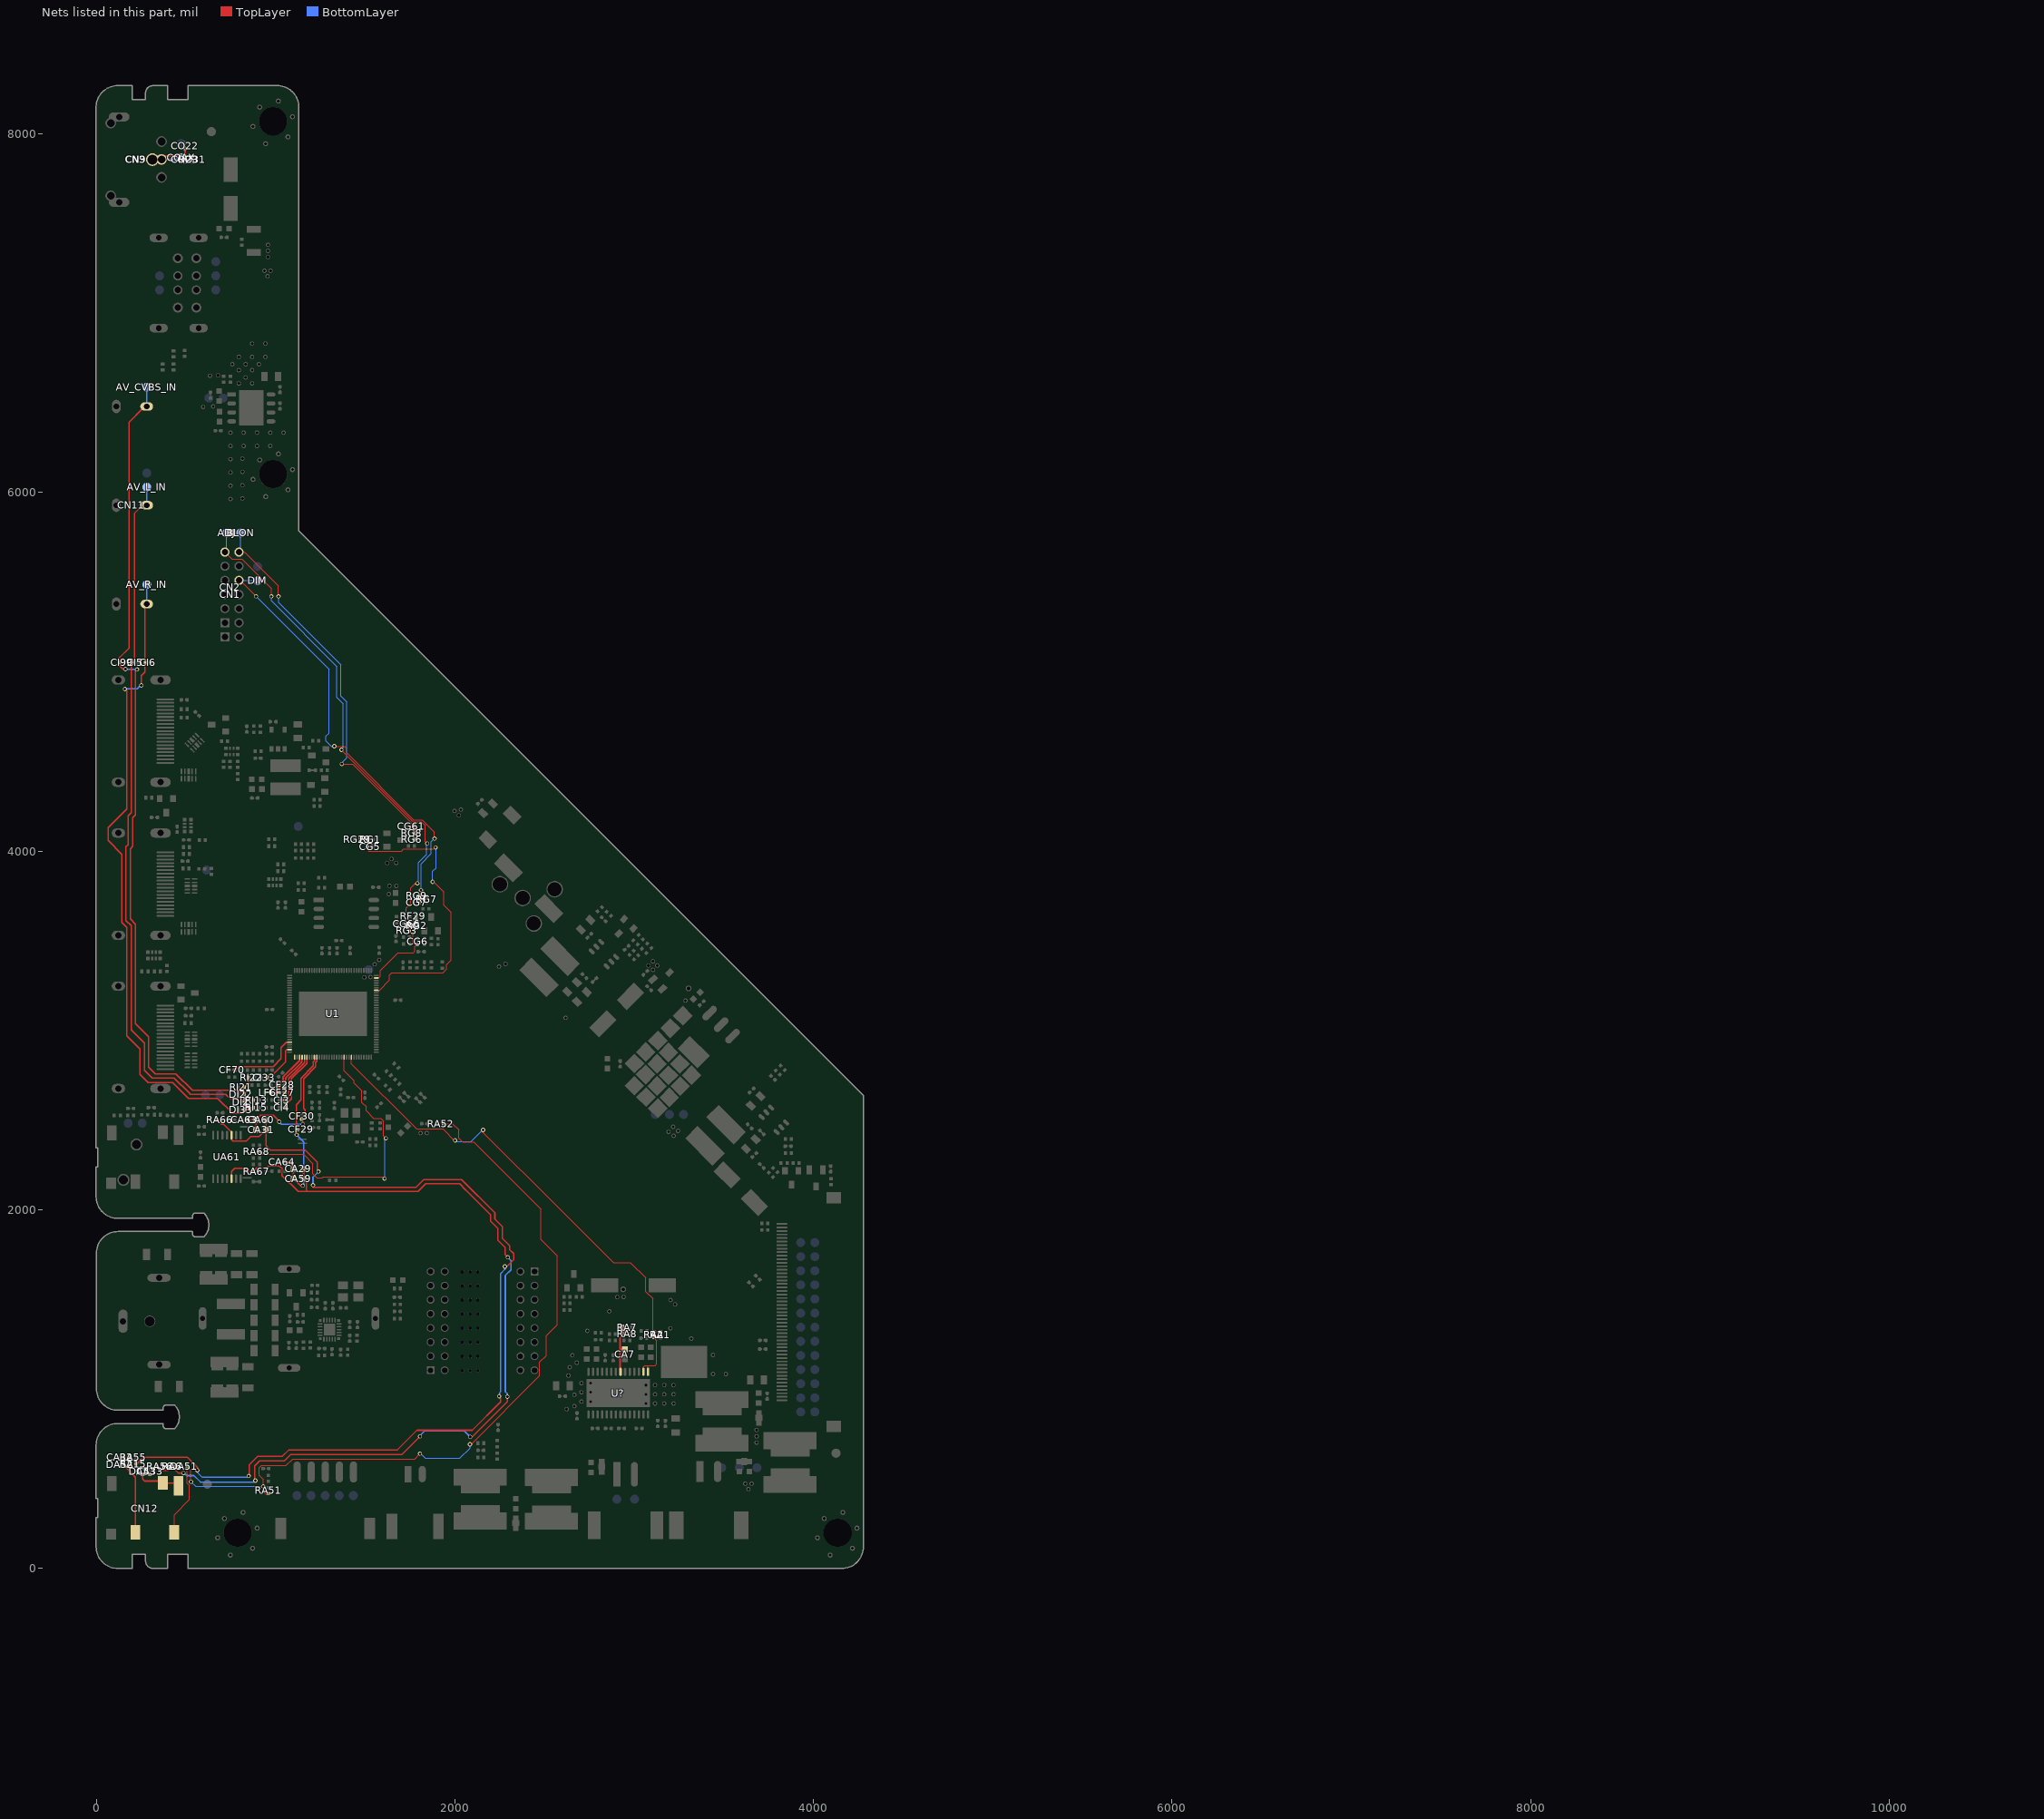
[diagram p0: the nets of this part, all layers, seen from the top]
# Altium PCB MISC105950.PcbDoc (part 6 of 15)
Units mil, origin at the board's own origin, x right, y up, seen from the top; angles counter-clockwise.
Board outline 4280.62 x 8272.76 mil, 2 copper layers (TopLayer, BottomLayer), stack 61.855 mil thick; 541 components, 268 nets, 2324 pads, 1157 vias.

## Via types
v1: diameter 23.62, hole 15.75, TopLayer to BottomLayer, tented both sides, 1087 vias
v2: diameter 23.62, hole 15.75, TopLayer to BottomLayer, 51 vias
v3: diameter 27.56, hole 19.68, TopLayer to BottomLayer, 15 vias
v4: diameter 31.5, hole 19.68, TopLayer to BottomLayer, tented both sides, 4 vias

## Nets (pads, with @x,y where several pads share a name; then routed paths per layer and width w, separated by ;. In a path a pad name is that pad's centre, name@x,y a point inside that pad or via, vN(x,y) a via of type N, cw(c..) or ccw(c..) an arc to the next point about the centre after c; other vN are vias at no path point) (continued)
ADIM: CG7.2@1795.85,3714 CG7.2@1802.74,3714 CN1.10 CN2.8 DIM.1 RG7.1 RG9.2 | length 2514.3
  TopLayer w5: CN2.8@794.34,5510.06 799.94,5510.06 v1(889.5,5420.5) ; v1(1326.5,4584.5) 1382,4584.5 1393.5,4573 1393.5,4549.61 1769.11,4174 1815.14,4174 1885,4104.14 v1@1885,4072 ; CG7.2@1802.74,3714 1803.23,3714.5 RG9.2@1803.23,3752 ; v1(1810,3782) 1810,3752 RG9.2@1803.23,3752 ; RG7.1@1841,3747.23 1836.23,3752 RG9.2@1803.23,3752
  BottomLayer w5: CN2.8@794.34,5510.06 897.01,5510.06 DIM.1@898.43,5508.64 ; v1(889.5,5420.5) 1296.5,5013.5 1296.5,4657.37 1279.69,4640.56 1279.69,4614.81 1310,4584.5 v1(1326.5,4584.5) ; v1(1810,3782) 1810,3928.5 1866.96,3985.46 1866.96,4050.96 v1(1885.5,4069.5)
ADIM_OUT_IC: CG5.2@1508.76,4024 CG5.2@1515.65,4024 RG1.2 RG29.1 U1.90 | length 1687
  TopLayer w5: RG29.1@1472.23,4064.5 RG1.2@1510.77,4064.5 CG5.2@1510.77,4026 ; CG5.2@1508.76,4024 1508.76,4008.24 1517,4000 1701.36,4000 1711.86,4010.5 1882,4010.5 v1(1891.5,4020) ; U1.90@1560.66,3222.78 1577.7,3222.78 1633.94,3279.02 1633.94,3293.19 1633.94,3309.19 1645.25,3320.5 1694.91,3320.5 1695,3320.4 1724,3320.4 1724.09,3320.5 1931.54,3320.5 1952.5,3341.46 1952.5,3365.22 1978.31,3391.03 1978.31,3656.47 1936.5,3698.28 1936.5,3771.14 1879.14,3828.5 v1(1874.5,3828.5) v1@1874.56,3828.44
  BottomLayer w5: v1(1874.5,3828.5) 1874.5,3886.5 1893.31,3905.31 v1@1893.31,4018.19
ADJ/PWM: ADJ.1 CG66.2@1738.85,3595 CG66.2@1745.74,3595 CN1.13 CN2.11 RG3.1 | length 2856.5
  TopLayer w5: CN2.11@715.6,5667.54 754.65,5628.5 812,5628.5 975,5465.5 v1(975,5420.5) ; v1@1366,4562.96 1764.96,4164 1811,4164 1832.69,4142.31 1832.69,4051.31 v1@1848,4036 ; RG3.1@1745.73,3555.5 CG66.2@1745.74,3595 1745.74,3611.22 1728.5,3628.46 1728.5,3682 1752.91,3706.41 1752.91,3787.5 1753.19,3787.77 1753.19,3793.5 ; v1@1789,3819.5 1779.19,3819.5 1753.19,3793.5 ; v1(1789.5,3820) 1789.5,3829.81 1753.19,3793.5
  BottomLayer w5: CN2.11@724.76,5676.7 ADJ.1@724.76,5772.46 ; v1(975,5420.5) 975,5396.52 1341.28,5030.24 1341.28,4856.91 1375.5,4822.69 1375.5,4576.5 v1@1366,4567 ; v1@1796,3826.5 1796,3935 1842.5,3981.5 v1@1842.5,4039.84
  other v1: 1844.5,4042 1366,4565
AMP_L_OUT_IC: CA29.1 CA59.1 CA64.1 CF29.1 U1.41 | length 1132.5
  TopLayer w7: CA64.1@1051.73,2262.41 CA64.1@1051.73,2266 1091.5,2266 1098.17,2259.33 CA29.1@1098.17,2226.34 CA59.1@1098.17,2172.75 1137.92,2133 v1(1150.5,2133) ; v1(1116,2416.5) 1113.69,2418.81 1113.69,2584.75 1140,2611.06 1140,2731 1209.82,2800.82 1209.82,2824.18 1215.15,2829.52 U1.41@1215.15,2849.72
  BottomLayer w7: v1(1116,2416.5) 1154.5,2378 1154.5,2301 ; v1(1150.5,2133) 1154.5,2137 1154.5,2186.5 ; 1154.5,2174.5 1154.5,2186.5 ; 1154.5,2192.5 1154.5,2301 ; 1154.5,2327.5 1154.5,2301 ; 1154.5,2186.5 1154.5,2301
AMP_MUTE_OUT: RA2.1 U?.1 U?.2 | length 295
  TopLayer w5: U?.2@3050.95,1094.5 3050.95,1122.45 3057.94,1129.44 3115.94,1129.44 3125.5,1139 3125.5,1268.27 RA2.1@3109,1284.77 ; U?.1@3076.54,1094.5 3076.54,1127.5
AMP_MUTE_OUT_IC: RA1.1 RA2.2 U1.56 | length 2607.4
  TopLayer w5: U1.56@1421.85,2849.72 1421.85,2812.98 1785.83,2449 1931.5,2449 v1@1997.5,2383 ; v1(2156,2444) 2156,2430.59 2584.34,2002.25 2585.91,2002.25 2883.67,1704.5 2978.7,1704.5 3063,1620.2 3063,1542.5 3102.95,1502.55 3102.95,1401.5 ; 3102.95,1373.86 3102.95,1401.5 ; RA1.1@3145,1318.23 RA2.2@3109,1318.23 3102.95,1324.28 3102.95,1401.5
  BottomLayer w5: v1@2007,2378.5 2090.5,2378.5 v1(2156,2444)
  other v1: 2000,2385.5
AMP_R_OUT_IC: CA31.1 CA60.1 CA63.1 CF30.1 U1.42 | length 829.4
  TopLayer w7: CA63.1@841.5,2501 888.56,2501 CA60.1@889.56,2500 ; CA60.1@889.31,2499.75 CA60.1@889.56,2500 ; CA31.1@889.81,2445 889.81,2499.75 CA60.1@889.56,2500 ; v1(1018.5,2489) 1018.5,2493.72 986.57,2525.66 915.22,2525.66 CA60.1@889.56,2500 ; v1@1150.5,2482 v1(1150.5,2475.5) 1150.5,2497.5 CF30.1@1144.5,2503.5 1152.23,2503.5 1163,2514.27 1163,2555.5 1154.5,2564 1154.5,2728.53 1221.82,2795.85 1221.82,2819.21 1228.93,2826.33 U1.42@1228.93,2849.72
  BottomLayer w7: v1(1018.5,2489) 1018.5,2488 1031,2475.5 v1(1150.5,2475.5)
AUVAG: CF27.2@1044.84,2652.5 CF27.2@1051.73,2652.5 CF28.2@1044.84,2694.5 CF28.2@1051.73,2694.5 U1.36 | length 226.8
  TopLayer w8: 1142.38,2820.35 1146.26,2824.23 U1.36@1146.26,2849.72
  TopLayer w10: CF27.2@1051.73,2652.5 CF28.2@1051.73,2694.5 ; CF28.2@1054.81,2702.75 1054.81,2732.79 1142.38,2820.35
AUVRM: CF27.1 CF28.1 LF6.2 LF6.3 U1.35 | length 283.3
  TopLayer w8: 1130.76,2828.54 1132.48,2830.25 U1.35@1132.48,2849.72
  TopLayer w10: LF6.2@979.47,2652.5 CF27.1@1018.27,2652.5 CF28.1@1018.27,2694.5 1018.27,2698.77 1039.81,2720.31 1039.81,2737.59 1130.76,2828.54
AV1_CVBS_IN_IC: CI33.2@945.35,2736.5 CI33.2@952.24,2736.5 U1.31 | length 225.1
  TopLayer w8: CI33.2@952.24,2736.5 972.96,2757.22 987.78,2757.22 1053.56,2823 1053.56,2885.44 1060.2,2892.07 U1.31@1076.34,2892.07
AV_CVBS_IN: AV_CVBS_IN.1 CI99.2@126.76,5052 CI99.2@133.65,5052 CN11.1 DI22.K RI21.2 RI22.1 | length 4729.1
  TopLayer w7: CI99.2@133.65,5052 128.27,5046.61 128.27,5034.23 147.5,5015 v1(161,5015) ; 217.31,4996.81 217.31,4984.5 ; v1(226,5013) 218.5,5013 217.31,5011.81 217.31,4984.5 ; RI21.2@823.73,2682.5 RI21.2@823.73,2679.48 ; RI22.1@847.77,2736.5 847.77,2703.51 RI21.2@823.73,2679.48 ; 217.31,4984.5 217.31,4201 202,4185.69 202,4025.78 188.5,4012.28 188.5,3620.78 216.5,3592.78 216.5,3036.78 290,2963.28 290,2794.5 327.21,2757.29 442.68,2757.29 535.28,2664.69 766,2664.69 766.53,2664.16 799.82,2664.16 822.35,2641.62 823.73,2643 RI21.2@823.73,2679.48
  TopLayer w8: CI99.2@126.76,5052 126.76,5078.26 180.5,5132 180.5,6392.31 254.57,6466.38 265.59,6466.38 CN11.1@279.53,6480.32
  BottomLayer w7: v1(161,5015) 163,5013 v1(226,5013) ; CN11.1@279.5,6480.35 AV_CVBS_IN.1@279.5,6588
AV_L_IN: AV_L_IN.1 CI5.2@200.26,5052 CI5.2@207.15,5052 CN11.3 DI2.K RI13.2 | length 4066.2
  TopLayer w7: CI5.2@200.26,5052 193.31,5045.05 193.31,4213.5 175,4195.19 175,4034 164.5,4023.5 164.5,3610.84 192.5,3582.84 192.5,3003 266,2929.5 266,2777 309.71,2733.29 432.74,2733.29 516.53,2649.5 523.34,2642.69 720.31,2642.69 720.56,2642.44 ; CI5.2@200.77,5052.5 CI5.2@200.77,5060.27
  TopLayer w8: CI5.2@200.26,5059.76 200.77,5060.27 200.77,5065.77 210.5,5075.5 210.5,5149.88 ; 210.5,5128.88 210.5,5149.88 ; CN11.3@279.53,5929.14 256.14,5929.14 210.5,5883.5 210.5,5149.88 ; 720.31,2642.19 743.67,2618.83 803.9,2618.83 DI2.K@823.73,2599 834.73,2610 RI13.2@875.77,2610
  BottomLayer w8: CN11.3@279.53,5929.14 280,5929.61 AV_L_IN.1@280,6030.37
AV_L_IN_IC: CI3.1 U1.37 | length 284.6
  TopLayer w7: CI3.1@1051.72,2610 1072,2630.28 1072,2730.88 1160.04,2818.92 U1.37@1160.04,2849.72
AV_R_IN: AV_R_IN.1 CI6.2@271.76,5052 CI6.2@278.65,5052 CN11.5 DI33.K RI15.2 | length 3690.7
  TopLayer w7: v1(158,4904) 168,4894 168,4234.5 63.5,4130 63.5,4058.5 140.5,3981.5 140.5,3600.9 168.5,3572.9 168.5,2968.78 242,2895.28 242,2755 287.71,2709.29 422.8,2709.29 511.4,2620.69 674.81,2620.69 759.5,2536 802.73,2536 DI33.K@823.23,2556.5 864.27,2556.5 RI15.2@875.77,2568 ; v1(249.62,4924.36) 249.62,4978.35 269.69,4998.42 CN11.5@269.69,5368.12 ; CI6.2@273.27,5046.61 CI6.2@278.65,5052
  TopLayer w8: CN11.5@269,5367.43 269.69,5368.12 CN11.5@279.53,5377.96
  BottomLayer w7: v1(158,4904) 227.63,4904 247.99,4924.36 v1(249.62,4924.36) ; CN11.5@280.5,5378.93 AV_R_IN.1@280.5,5486.87
AV_R_IN_IC: CI4.1 U1.38 | length 332.3
  TopLayer w7: CI4.1@1051.72,2568 1051.72,2581.87 1088,2618.15 1088,2729.91 1173.82,2815.73 U1.38@1173.82,2849.72
AVCC: CA7.2 RA7.2 RA8.1 U?.7 | length 302.2
  TopLayer w10: 2921.25,1266.75 2921.25,1248 ; U?.7@2923,1094.5 2921.25,1096.25 2921.25,1220.5 ; RA8.1@2942.77,1306.5 2921.25,1284.98 2921.25,1248 ; CA7.2@2947,1220.31 2921.44,1220.31 2921.25,1220.5 ; 2921.25,1220.5 2921.25,1248
  TopLayer w15: RA8.1@2942.77,1306.5 RA7.2@2942.77,1342.5
BL_ON: BLON.1 CG61.2@1763.85,4138.5 CG61.2@1770.74,4138.5 CN1.14 CN2.12 RG6.1 RG8.2 | length 2183.7
  TopLayer w5: CN2.12@794.34,5667.54 825.46,5667.54 1013,5480 1013,5422.5 v1(1015,5420.5) ; v1(1368.22,4485.24) 1428.52,4485.24 1773.23,4140.53 RG8.2@1773.23,4095.5 ; RG6.1@1775.73,4059.5 RG8.2@1775.73,4093
  BottomLayer w5: CN2.12@803.5,5676.7 BLON.1@803.5,5772.46 ; v1(1015,5420.5) 1015,5386.35 1362.28,5039.07 1362.28,4865.61 1396.5,4831.39 1396.5,4521.5 1368.22,4493.22 v1(1368.22,4485.24)
BRI_ADJ: CG6.2@1789.5,3478.76 CG6.2@1789.5,3485.65 RF29.1 RG2.2 U1.95 | length 576.9
  TopLayer w5: U1.95@1560.66,3291.68 1573.06,3291.68 1581.94,3300.56 1581.94,3333.55 1681.58,3433.19 1714.5,3433.19 ; 1695.58,3433.19 1714.5,3433.19 ; 1766.5,3503.76 1766.5,3525 ; RF29.1@1782.5,3639.77 1767.16,3624.43 1767.16,3585.61 RG2.2@1784.5,3568.27 1766.5,3550.27 1766.5,3525 ; CG6.2@1783.85,3480 1771.5,3480 1766.5,3485 1766.5,3525 ; CG6.2@1790,3480.26 1776.5,3466.76 1776.5,3441.5 1768.19,3433.19 1714.5,3433.19
COAX_OUT: CN3.1 CN9.2 CO22.2@493,7918.64 CO22.2@493,7925.53 CO23.2@493,7868.72 CO23.2@493,7875.61 COAX.1 RO31.1 | length 384.7
  TopLayer w10: CN3.1@307.08,7857.7 326,7876.61 493,7876.61 493.5,7876.61 RO31.1@528.5,7876.61
  TopLayer w12: CO23.2@493.5,7876.11 493.5,7876.61 CO22.2@493.5,7918.64
  BottomLayer w12: CN9.2@362.2,7858.27 460.5,7858.27 COAX.1@470.87,7868.64
CVBS_OUT_IC: U1.33
EPH_DET_IN: CN12.5 DA51.K RA51.1 RA52.1 | length 4675.5
  TopLayer w5: CN12.5@433.07,198.82 433.07,297.57 518.5,383 518.5,461 504.73,474.77 DA51.K@504.73,568.5 526.5,546.73 v2(526.5,481) ; RA51.1@957.5,415.77 940.73,415.77 929.5,427 v2(929.5,455) ; v1(1804,637.5) 1775.38,608.88 1093.53,608.88 1057.87,573.21 920.26,573.21 907,559.95 907,517.5 929.5,495 v2@929.5,457 ; RA52.1@1935.73,2478.5 1985.81,2478.5 2020.45,2443.86 2020.45,2397.55 2042,2376 2104.52,2376 2479.31,2001.21 2479.31,1831.73 2570.5,1740.54 2570.5,1357.33 2508.36,1295.19 2508.36,1184.86 2472.36,1148.86 2472.36,1073.57 v1@2088.45,689.65 ; v2(929.5,455) 931.5,455 v2@929.5,457 ; v2(929.5,455) v2@929.5,457
  BottomLayer w5: v2(526.5,481) 552.5,455 v2(929.5,455) ; v1@1809.44,637.5 1834.72,612.21 2025.97,612.21 2083.28,669.53 v1(2083.28,689.65)
EPH_L_OUT: CA29.2 CA59.2 RA6.1 RA67.2 UA61.12 | length 5076.7
  TopLayer w5: 1035.25,2200.14 1035.25,2227.74
  TopLayer w7: UA61.12@752.77,2171.5 752.77,2212.27 771,2230.5 820.5,2230.5 837.5,2213.5 RA67.2@875.77,2213.5 894.11,2231.84 947.37,2231.84 959.37,2243.84 1019.15,2243.84 1035.25,2227.74 ; 1035,2199.51 1035,2189.75 1124.55,2100.19 1792.9,2100.19 1835.55,2142.85 2025.14,2142.85 2059.13,2108.86 ; CA29.2@1153.79,2226.34 1153.79,2169.81 1171.11,2152.5 1171.11,2101.58
  TopLayer w8: RA6.1@437.23,567.5 437.23,548.27 455.5,530 v2(485,530) ; v2(885.5,487.5) 882.5,490.5 882.5,570.1 910.12,597.71 1047.72,597.71 1083.38,633.38 1702.88,633.38 v1(1804,734.5) ; 2059.48,2109.21 2197.34,1971.35 2197.34,1936.13 2239.19,1894.28 2239.19,1828.28 2278.69,1788.78 2278.69,1748.81 v1(2294,1733.5) ; 2096.15,732 2291.5,927.35 v1(2291.5,956)
  BottomLayer w8: v2(485,530) 487,530 501.5,515.5 543.38,515.5 579.38,479.5 877.5,479.5 v2(885.5,487.5) ; v1@1804,739.56 1829.53,765.09 2050.91,765.09 v1(2084,732) ; v1(2291.5,956) 2291.5,972.5 2280.5,983.5 2280.5,1632.2 2312,1663.7 2312,1715.5 v1(2294,1733.5)
EPH_LOUT: CA33.1 CN12.4 CN12.6 DA53.K RA6.2 RA56.2 | length 431.3
  TopLayer w8: RA6.2@403.77,567.5 403.77,549.27 398,543.5 355,543.5 339.48,559.02 339.48,563.29 RA56.2@335.77,567 322.5,553.73 322.5,530.5 313.77,521.77 CA33.1@297,521.77 256.99,521.77 DA53.K@256.5,522.27 256.5,496 267.5,485 359.49,485 CN12.4@370.08,474.41 CN12.6@439.96,474.41
EPH_R_OUT: CA31.2 CA60.2 RA15.1 RA66.2 UA61.3 | length 5506.6
  TopLayer w8: RA15.1@220.23,580.5 223.5,580.5 261.31,618.31 506.07,618.31 562,562.38 v2(562,545) ; RA66.2@670.77,2501 694.96,2476.81 707.3,2476.81 UA61.3@752.77,2431.34 ; UA61.3@752.77,2414.61 752.77,2389.23 760.5,2381.5 835,2381.5 861.31,2407.81 907.75,2407.81 CA31.2@944.94,2445 ; v2@851.69,516.69 851.69,576.06 899.35,623.71 1036.95,623.71 1072.61,659.38 1678.38,659.38 1787.35,768.35 2095.72,768.35 2253.81,926.43 v1@2253.81,949.69 ; CA60.2@944.94,2499.75 CA31.2@944.94,2445 ; v1@1207.5,2124.69 1782.75,2124.69 1825.41,2167.35 2036.7,2167.35 2222.34,1981.71 2222.34,1946.48 2264.19,1904.63 2264.19,1838.63 2303.69,1799.13 2303.69,1777.41 2327,1754.1 2327,1720.1 v1@2288.9,1682 ; v1@1230.61,2219.39 1230.61,2265.2 1163.96,2331.84 969.16,2331.84 944.94,2356.06 CA31.2@944.94,2445
  BottomLayer w8: v2(562,545) 562,533.65 590.15,505.5 840.5,505.5 v2(848.5,513.5) v2@850,512 ; v1(1207.5,2135.5) 1207.5,2180.5 v1(1238.5,2211.5) ; v1@2249,958 2249,978.23 2254.5,983.73 2254.5,1642.97 2278,1666.47 v1(2278,1682)
  other v1: 2245.5,958
EPH_ROUT: CA32.1 CN12.3 DA52.K RA15.2 RA55.2 | length 523.3
  TopLayer w7: RA15.2@186.77,580.5 RA55.2@186.77,618 149.23,618 CA32.1@148.23,617 148.23,576.99 DA52.K@147.73,576.5 180.62,543.62 216.54,507.7 CN12.3@216.54,198.82
EPH_SDN_OUT_IC: RA68.1 U1.53 | length 1641.5
  TopLayer w5: RA68.1@909.23,2323.75 924.64,2308.34 1154.23,2308.34 1207.11,2255.47 1207.11,2198.56 1229.17,2176.5 1258.06,2176.5 1263.56,2182 1599,2182 1606.5,2174.5 v1(1606.5,2172.5) ; U1.53@1379.16,2848.37 U1.53@1379.84,2849.05 ; U1.53@1380.51,2849.05 U1.53@1380.51,2849.72 U1.53@1379.84,2849.05 ; v1(1614,2397.5) 1601.45,2410.05 1601.45,2493.08 1585.43,2509.09 1546.4,2509.09 1503.5,2551.99 1503.5,2573.78 1479.66,2597.63 1479.66,2662.07 1435.2,2706.53 1435.2,2717.6 1379.84,2772.96 U1.53@1379.84,2849.05
  BottomLayer w5: v1(1606.5,2172.5) 1609,2175 1609,2225.5 ; 1609,2188 1609,2225.5 ; v1(1614,2397.5) 1609,2397.5 1609,2225.5
GIN1N: CF70.1 U1.28 | length 404.8
  TopLayer w7: CF70.1@771.73,2779 789.88,2797.15 985,2797.15 1029.06,2841.22 1029.06,2903.14 1059.34,2933.41 U1.28@1076.34,2933.41